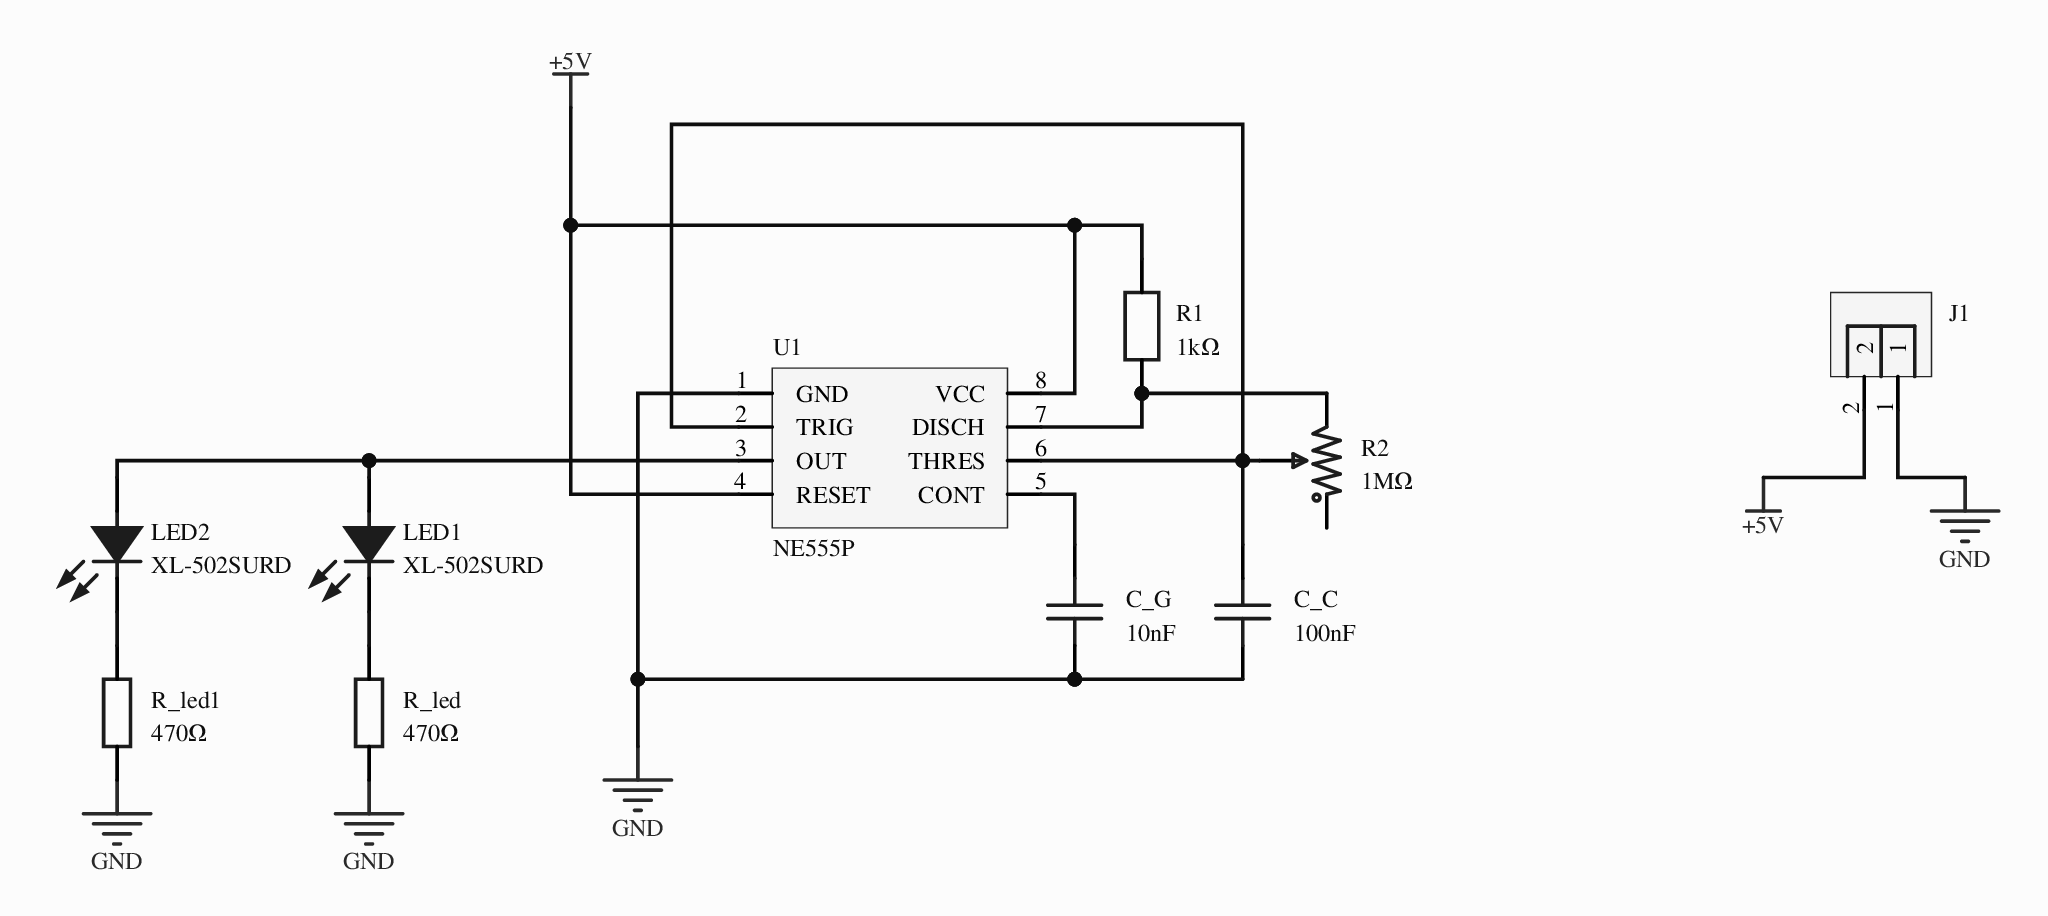
[diagram p0: MISC49908-3.schdoc]
# Altium project MISC49908-2.PrjPcb
1 sheet, 10 parts. Net scope: global (net labels, ports and power ports of the same name join across sheets).
Board file: MISC49908.pcbdoc

## Sheet MISC49908-3.schdoc
size 210 x 148 mm; Version: V1.0; @Project Name: MISC49908; @Update Date: 2026-10-07; @Create Date: 2026-10-07; @Board Name: MISC49908; @Create Time: 12:44:54; @Page Count: 1; @Page No: 1; @Schematic Name: MISC49908; @Update Time: 12:44:54; Size: A4

### Parts
C_C  100nF  [CAP-TH_L5.0-W2.5-P5.00-D1.0]
C_G  10nF  [CAP-TH_L5.5-W3.0-P5.00-D0.6]
J1  (no value)  [HDR-TH_2P-P2.54-V-M-1]
LED1  XL-502SURD  [LED-TH_BD5.9-P2.54-RD_RED]
LED2  XL-502SURD  [LED-TH_BD5.9-P2.54-RD_RED]
R1  1kΩ  [RES-TH_BD2.7-L6.2-P10.20-D0.4]
R2  1MΩ  [RES-ADJ-TH_RM063-103]
R_led  470Ω  [RES-TH_BD2.3-L6.5-P10.50-D0.5]
R_led1  470Ω  [RES-TH_BD2.3-L6.5-P10.50-D0.5]
U1  NE555P  [DIP-8_L9.8-W6.6-P2.54-LS7.6-BL]

### Nets
+5V: J1.2 R1.2 U1.4(RESET) U1.8(VCC)
GND: C_C.1 C_G.1 J1.1 R_led.1 R_led1.1 U1.1(GND)
NetC_C_2: C_C.2 R2.2 U1.2(TRIG) U1.6(THRES)
NetC_G_2: C_G.2 U1.5(CONT)
NetLED1_1: LED1.1(K) R_led.2
NetLED1_2: LED1.2(A) LED2.2(A) U1.3(OUT)
NetLED2_1: LED2.1(K) R_led1.2
NetR1_1: R1.1 R2.3 U1.7(DISCH)

Not connected (* = marked no-connect by the designer): R2 1*

### Library data of the parts
C_C = CC1H104MC1FD3F6C10MF: Capacitance: 100nF; tolerance: ±20%; rated voltage: 50V; temperature coefficient: Y5V;; Manufacturer: Dersonic(德尔创); 3D Model: 08e3d7481fc7486bb1b263873f51e1e10819f05c4eef4c71ace90d822a990e87; 3D Model Transform: 224.652,98.425,0,0,0,0,-0.005,0,-137.795; Pin Spacing: 5.08mm; Body Thickness: 2.2mm; AddInBom: yes; ModelName: CAP-TH_BD5.0-W2.5-P5.08; Symbol: CC1H104MC1FD3F6C10MF; Device: CC1H104MC1FD3F6C10MF; LCSC Part Name: 100nF ±20% 50V; Supplier Part: C254085; Manufacturer Part: CC1H104MC1FD3F6C10MF; Supplier Footprint: 插件,P=5.08mm; JLCPCB Part Class: Extended Part; Supplier: LCSC; Value: 100nF; Tolerance: ±20%; Voltage Rating: 50V; Temperature Coefficient: Y5V; Diameter: 6mm; FootprintName: CAP-TH_L5.0-W2.5-P5.00-D1.0; ConvertToPcb: yes
C_G = DCT103M22Y5UF6FJ5A0: Capacitance: 10nF; tolerance: ±20%; rated voltage: 50V; temperature coefficient: Y5U;; Manufacturer: SHM(南方宏明); 3D Model: 8f31db7ace7a416e97923e9ed245e9d50819f05c4eef4c71ace90d822a990e87; 3D Model Transform: 232.661,127.248,0,0,0,0,-0.005,0,-196.85; Pin Spacing: 5mm; AddInBom: yes; Symbol: DCT103M22Y5UF6FJ5A0; Device: DCT103M22Y5UF6FJ5A0; LCSC Part Name: 10nF ±20% 50V; Supplier Part: C2896035; Manufacturer Part: DCT103M22Y5UF6FJ5A0; Supplier Footprint: 插件,P=5mm; JLCPCB Part Class: Extended Part; Supplier: LCSC; Value: 10nF; Tolerance: ±20%; Voltage Rating: 50V; Temperature Coefficient: Y5U; FootprintName: CAP-TH_L5.5-W3.0-P5.00-D0.6; ConvertToPcb: yes; ModelName: CAP-TH_L5.5-W3.0-P5.00-D0.6
J1 = HDR-M_2.54_1x2P: Symbol: 210S-1*2P L=11.6MMGold-plated black; 3D Model: 79b2e9f2d70a4d68a1b7098f27c6d4c50819f05c4eef4c71ace90d822a990e87; 3D Model Transform: 200,100,0,0,0,0,0,0,-118.11; ConvertToPcb: yes; ModelName: HDR-M-2.54_1x2; Device: HDR-M_2.54_1x2P; Supplier Part: C124375; Supplier Footprint: 插件; FootprintName: HDR-TH_2P-P2.54-V-M-1; AddInBom: yes
LED1 LED2 = XL-502SURD: Lamp holder type: 5mm round lamp holder; illumination colour: red; forward voltage (Vf): 2.4V; power: 70mW; forward current: 20mA; wavelength: 615nm~625nm; diode configuration: -; lens colour: red lens; colour temperature: -; luminous intensity: 300mcd; viewing angle: 35°; tape packaging: -; operating temperature: -25℃~+85℃;; Manufacturer: XINGLIGHT(成兴光); 3D Model: fe9cea1bdf7642cd8d9a5077ed0e2b580819f05c4eef4c71ace90d822a990e87; 3D Model Transform: 211.96686,228.01584,0,0,0,0,7.874,0,-137.795; Peak Wavelength: 654nm; AddInBom: yes; Symbol: XL-502SURD; Device: XL-502SURD; LCSC Part Name: 5mm圆形灯头 红色; Supplier Part: C2895492; Manufacturer Part: XL-502SURD; Supplier Footprint: 插件,D=5mm; JLCPCB Part Class: Extended Part; Supplier: LCSC; Lamp Holder Type: 5mm round lamp holder; Illumination Color: Red; Voltage - Forward(Vf): 2.4V; Power(Watts): 70mW; Forward Current: 20mA; Wavelength - Dominant: 615nm~625nm; Diode Configuration: -; Lens Color: Red lens; Color Temperature: -; Luminous Intensity: 300mcd; Viewing Angle: 35°; Mounting Style: -; Operating Temperature: -25℃~+85℃; FootprintName: LED-TH_BD5.9-P2.54-RD_RED; ConvertToPcb: yes; ModelName: LED-TH_BD5.9-P2.54-RD_RED
R1 = MF1/4W-1K±1%-ST52: Resistor type: metal film resistor; resistance: 1kΩ; tolerance: ±1%; power: 250mW; temperature coefficient: ±100ppm/℃;; Manufacturer: VO(翔胜); 3D Model: f91fbe0e2e6f409498f09f811e4616fe0819f05c4eef4c71ace90d822a990e87; 3D Model Transform: 417.322,106.221,0,0,0,0,0,0,-196.85; Voltage-Supply(Max): 250V; AddInBom: yes; Symbol: MF1/4W-1K±1%-ST52; Device: MF1/4W-1K±1%-ST52; LCSC Part Name: 金属膜电阻 1kΩ ±1% 250mW; Supplier Part: C2903245; Manufacturer Part: MF1/4W-1K±1%-ST52; Supplier Footprint: 插件,D2.7xL6.2mm; JLCPCB Part Class: Extended Part; Supplier: LCSC; Type: Metal film resistor; Value: 1kΩ; Tolerance: ±1%; Power(Watts): 250mW; Temperature Coefficient: ±100ppm/℃; Operating Temperature: -55℃~+155℃; FootprintName: RES-TH_BD2.7-L6.2-P10.20-D0.4; ConvertToPcb: yes; ModelName: RES-TH_BD2.7-L6.2-P10.20-D0.4
R2 = RM063-105(1M): Resistance: 1MΩ; tolerance: ±25%; power: 100mW;; Manufacturer: BOCHEN(博晨); 3D Model: c2e79538aa8f4a14bd3d91be27bc95d30819f05c4eef4c71ace90d822a990e87; 3D Model Transform: 255.905,230.194,0,0,0,0,0,-52.48,-137.795; Voltage Rating: 50V; AddInBom: yes; Symbol: RM063-105(1M); Device: RM063-105(1M); LCSC Part Name: 1MΩ ±25%; Supplier Part: C5205038; Manufacturer Part: RM063-105(1M); Supplier Footprint: 插件,6.4x5.2mm; JLCPCB Part Class: Extended Part; Datasheet: )/5896396.html; Supplier: LCSC; Value: 1MΩ; Tolerance: ±25%; Power(Watts): 100mW; FootprintName: RES-ADJ-TH_RM063-103; ConvertToPcb: yes; ModelName: RES-ADJ-TH_RM063-103
R_led R_led1 = MF1/2WS-470Ω±1% T: Resistor type: metal film resistor; resistance: 470Ω; tolerance: ±1%; power: 500mW; temperature coefficient: ±100ppm/℃;; Manufacturer: CCO(千志电子); Symbol: MF1/2WS-470Ω±1% T52; 3D Model: 8e6c7ee8323443d1ab8f0504b6353c8c0819f05c4eef4c71ace90d822a990e87; 3D Model Transform: 431.1015,91.3384,0,0,0,0,0.197,0,-137.795; Voltage-Supply(Max): 250V; AddInBom: yes; ModelName: RES-TH_D2.3-L6.5-P10.50; Device: MF1/2WS-470Ω±1% T; LCSC Part Name: 470Ω ±1% 500mW 金属膜电阻 小体积,p;-[[圆柱直插; Supplier Part: C129899; Manufacturer Part: MF1/2WS-470Ω±1% T; Supplier Footprint: 插件,D2.3xL6.5mm; JLCPCB Part Class: Extended Part; Supplier: LCSC; Type: Metal film resistor; Value: 470Ω; Tolerance: ±1%; Power(Watts): 500mW; Temperature Coefficient: ±100ppm/℃; Operating Temperature: -55℃~+155℃; FootprintName: RES-TH_BD2.3-L6.5-P10.50-D0.5; ConvertToPcb: yes
U1 = NE555P: These devices are precision timing circuits that generate accurate time delays or oscillations. In delay or monostable mode, the timing interval is controlled by a single external resistor and capacitor network. In astable mode, the frequency and duty cycle can be controlled separately by two external resistors and one external capacitor.; Manufacturer: TI(德州仪器); 3D Model: db2af726fcec488f8bf8e467aca974b30819f05c4eef4c71ace90d822a990e87; 3D Model Transform: 385.826,311.8104,0,0,0,0,-1.693,0,-137.795; AddInBom: yes; ModelName: DIP-8_L9.8-W6.6-H3.5-LS7.62-P2.54; Symbol: NE555P; Device: NE555P; LCSC Part Name: NE555P; Supplier Part: C46749; Manufacturer Part: NE555P; Supplier Footprint: DIP-8; JLCPCB Part Class: Extended Part; Supplier: LCSC; FootprintName: DIP-8_L9.8-W6.6-P2.54-LS7.6-BL; ConvertToPcb: yes